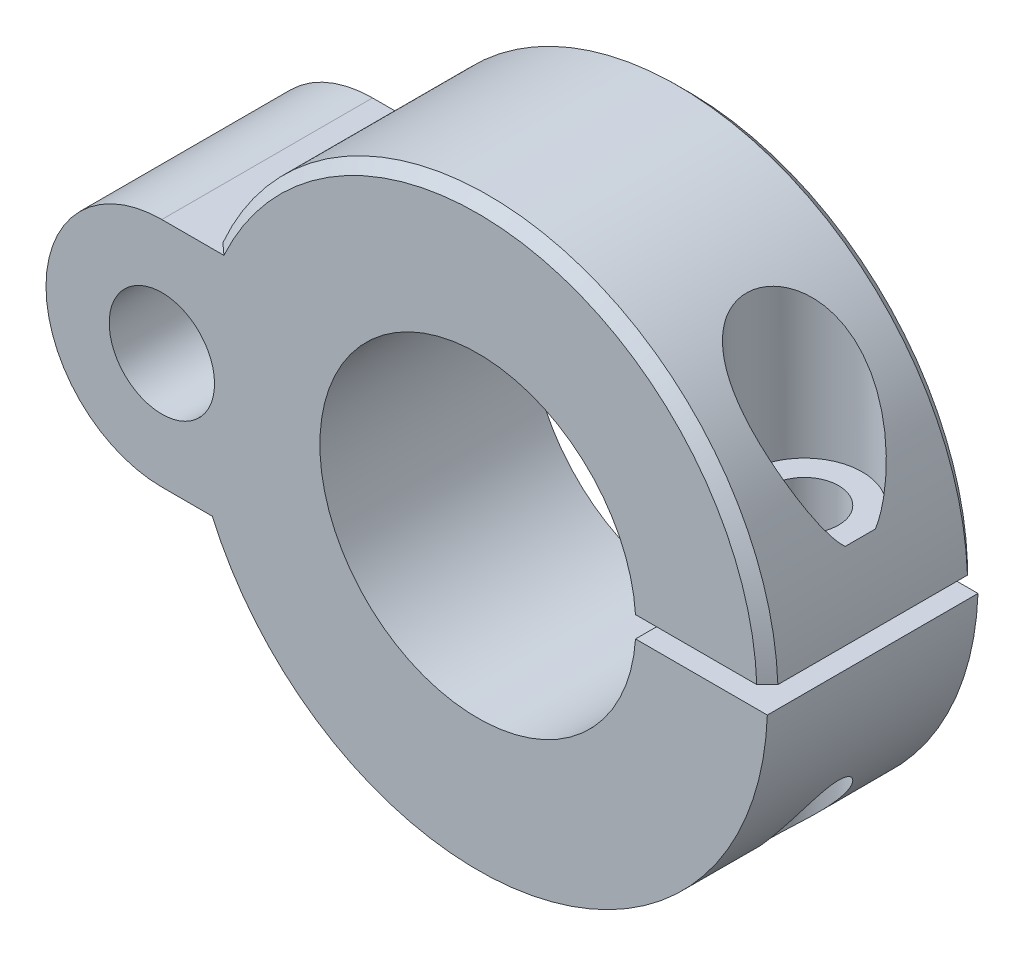
SolidWorks part; units mm, degrees
ref_plane "前视基准面" through (0, 0, 0) normal (0, 0, 1) x (1, 0, 0)
ref_plane "上视基准面" through (0, 0, 0) normal (0, 1, 0) x (1, 0, 0)
ref_plane "右视基准面" through (0, 0, 0) normal (1, 0, 0) x (0, 0, -1)
ref_plane "基准面4" through (0, 0, 10) normal (0, 0, 1) x (1, 0, 0)
sketch "草图1" plane through (0, 0, 10) normal (0, 0, 1) x (1, 0, 0)
  line L0 (-25.2042, 11) -> (-30, 11)
  line L1 (-30, -11) -> (-25.2042, -11)
  arc A0 (-25.2042, -11) -> (-25.2042, 11) centre (0, 0) ccw
  arc A1 (-30, 11) -> (-30, -11) centre (-30, 0) ccw
extrude "凸台-拉伸1" add sketch "草图1" against normal blind 20
sketch "草图2" plane through (0, 0, -10) normal (0, 0, -1) x (-1, 0, 0)
  line L0 (-27.4818, -1) -> (-14.9666, -1)
  line L1 (-14.9666, 1) -> (-27.4818, 1)
  arc A0 (-27.4818, 1) -> (-27.4818, -1) centre (0, 0) ccw
  arc A1 (-14.9666, -1) -> (-14.9666, 1) centre (0, 0) cw
extrude "切除-拉伸1" cut sketch "草图2" against normal through all
ref_plane "基准面5" through (0, 0, 0) normal (0, -1, 0) x (1, 0, 0)
sketch "草图3" plane through (0, 0, 0) normal (0, -1, 0) x (1, 0, 0)
  line L0 (15, 10) -> (0, 10)
  line L1 (0, 10) -> (0, -10)
  line L2 (0, -10) -> (15, -10)
  line L3 (15, -10) -> (15, 10)
  line L4 (0, 10) -> (0, -10) construction
revolve "切除-旋转1" cut sketch "草图3" angle 360 about L4
hole_wizard "Ø10.0 (10) 直径孔1" positions "草图5" profile "草图4" hole size "Ø10.0" standard "ANSI Metric"
sketch "草图5" plane through (0, 0, 10) normal (0, 0, 1) x (1, 0, 0)
  point P0 (-30, 0)
sketch "草图4" plane through (-30, 0, 10) normal (1, 0, 0) x (0, -1, 0)
  line L0 (0, 0) -> (0, 20)
  line L1 (0, 20) -> (5, 20)
  line L2 (5, 20) -> (5, 0)
  line L5 (5, 0) -> (0, 0)
  line L11 (0, -6.35) -> (0, 107.95) construction
  dimension "通孔孔直径" = 10
  dimension "通孔孔深度" = 20
hole_wizard "Ø5.0 (5) 直径孔1" positions "草图7" profile "草图6" hole size "Ø5.0" standard "ANSI Metric"
sketch "草图7" plane through (0, -1, 0) normal (0, 1, 0) x (1, 0, 0)
  point P0 (21, 0)
sketch "草图6" plane through (21, -1, 0) normal (1, 0, 0) x (0, 0, 1)
  line L0 (0, 0) -> (0, 26.5)
  line L1 (0, 26.5) -> (2.5, 26.5)
  line L2 (2.5, 26.5) -> (2.5, 0)
  line L5 (2.5, 0) -> (0, 0)
  line L11 (0, -6.35) -> (0, 107.95) construction
  dimension "通孔孔直径" = 5
  dimension "通孔孔深度" = 26.5
ref_plane "基准面6" through (0, 22.7156, 0) normal (0, 1, 0) x (1, 0, 0)
hole_wizard "M6 六角头螺栓的柱形沉头孔1" positions "草图9" profile "草图8" counterbore size "M6" standard "ANSI Metric"
sketch "草图9" plane through (0, 22.7156, 0) normal (0, 1, 0) x (1, 0, 0)
  point P0 (21, 0)
sketch "草图8" plane through (21, 22.7156, 0) normal (1, 0, 0) x (0, 0, 1)
  line L0 (0, 0) -> (0, 50.2156)
  line L1 (0, 50.2156) -> (3.25, 50.2156)
  line L3 (3.25, 50.2156) -> (3.25, 14.7156)
  line L4 (3.25, 14.7156) -> (5.5, 14.7156)
  line L5 (5.5, 14.7156) -> (5.5, 0)
  line L7 (5.5, 0) -> (0, 0)
  line L11 (0, -6.35) -> (0, 107.95) construction
  dimension "通孔孔直径" = 6.5
  dimension "通孔孔深度" = 50.2156
  dimension "柱形沉头孔直径" = 11
  dimension "柱形沉头孔深度" = 14.7156
chamfer "倒角1" distance 1 angle 45 2 edges at (5.1281, 27.0176, -10) (5.1281, 27.0176, 10)
